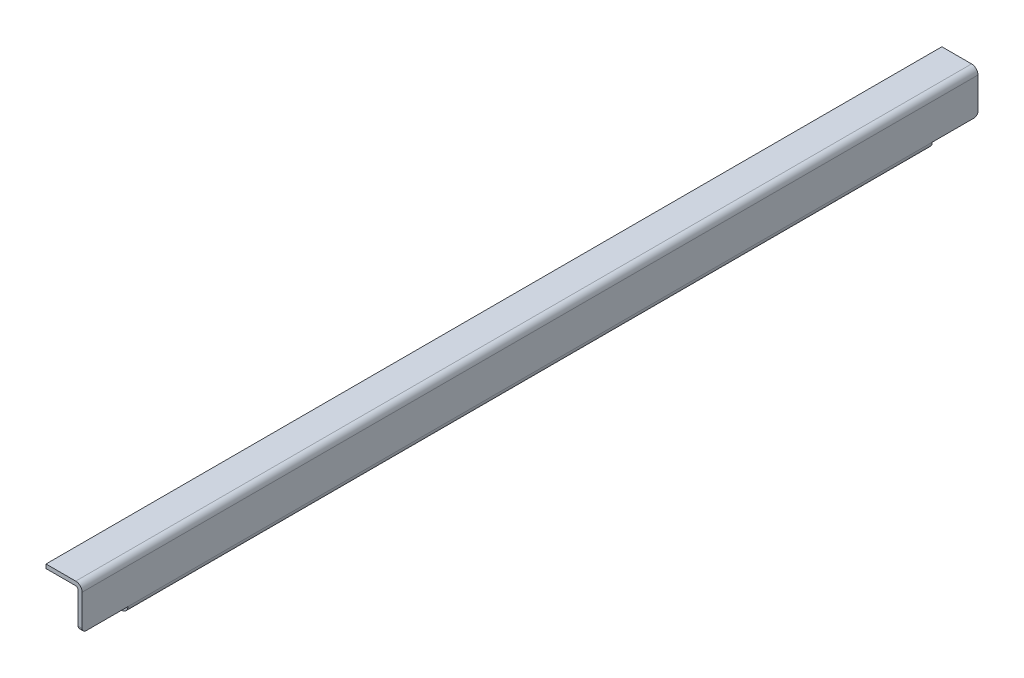
from build123d import *

# Parameters (mm, degrees)
BOSS_EXTRUDE1_DEPTH    = 1116
SKETCH2_W              = 92.475127077
SKETCH2_H              = 38.646657261
SKETCH2_W_2            = 90.397253408
SKETCH2_H_2            = 44.857464027
CUT_EXTRUDE1_DEPTH     = 1116
SKETCH3_R              = 4
CUT_EXTRUDE2_DEPTH     = 1116
FILLET1_R              = 5
M10_TAPPED_HOLE1_D     = 8.5
M10_TAPPED_HOLE1_DEPTH = 24.5
M10_TAPPED_HOLE1_TIP   = 2.553657631


with BuildPart() as part:
    # Sketch1 → Boss-Extrude1 (new body)
    with BuildSketch(Plane.XY):
        with BuildLine():
            Line((0, 0), (37, 0))
            ThreePointArc((37, 0), (42.656854249, -2.343145751), (45, -8))
            Line((45, -8), (45, -52))
            ThreePointArc((45, -52), (42.656854249, -57.656854249), (37, -60))
            Line((37, -60), (0, -60))
            Line((0, -60), (0, -55))
            Line((0, -55), (37, -55))
            ThreePointArc((37, -55), (39.121320344, -54.121320344), (40, -52))
            Line((40, -52), (40, -8))
            ThreePointArc((40, -8), (39.121320344, -5.878679656), (37, -5))
            Line((37, -5), (0, -5))
            Line((0, -5), (0, 0))
        make_face()
    extrude(amount=BOSS_EXTRUDE1_DEPTH)

    # Sketch2 → Cut-Extrude1 (cut)
    with BuildSketch(Plane.ZY):
        with Locations((1105.237563539, -71.323328631)):
            Rectangle(SKETCH2_W, SKETCH2_H)
        with Locations((11.801373296, -74.428732013)):
            Rectangle(SKETCH2_W_2, SKETCH2_H_2)
    extrude(amount=-CUT_EXTRUDE1_DEPTH, mode=Mode.SUBTRACT)

    # Sketch3 → Cut-Extrude2 (cut)
    with BuildSketch(Plane(origin=(0, -55, 0), x_dir=(1, 0, 0), z_dir=(0, 1, 0))):
        with Locations(Location((12.5, -1024, 0), (0, 0, 270))):
            Circle(SKETCH3_R)
    extrude(amount=-CUT_EXTRUDE2_DEPTH, mode=Mode.SUBTRACT)

    # Fillet1
    fillet1_edges = [part.edges().sort_by_distance(p)[0] for p in [
        (42.5, -52, 0),
        (42.5, -52, 1116),
    ]]
    fillet(fillet1_edges, radius=FILLET1_R)

    # M10 Tapped Hole1
    with Locations(Plane(origin=(0, -55, 0), x_dir=(1, 0, 0), z_dir=(0, 1, 0))):
        with Locations((12.5, -1024)):
            Hole(M10_TAPPED_HOLE1_D / 2, depth=M10_TAPPED_HOLE1_DEPTH)
            with Locations((0, 0, -(M10_TAPPED_HOLE1_DEPTH + M10_TAPPED_HOLE1_TIP / 2))):  # 118° drill point
                Cone(0, M10_TAPPED_HOLE1_D / 2, M10_TAPPED_HOLE1_TIP, mode=Mode.SUBTRACT)


solid = part.part
